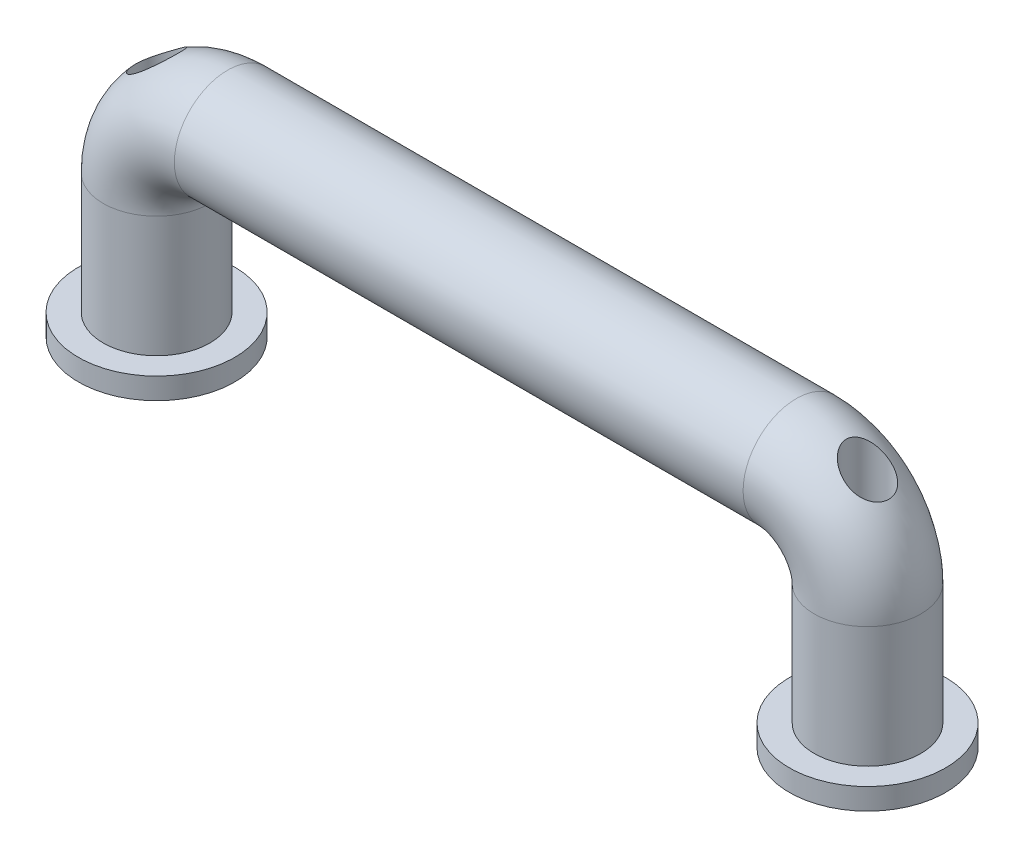
SolidWorks part; units mm, degrees
ref_plane "前视基准面" through (0, 0, 0) normal (0, 0, 1) x (1, 0, 0)
ref_plane "上视基准面" through (0, 0, 0) normal (0, 1, 0) x (1, 0, 0)
ref_plane "右视基准面" through (0, 0, 0) normal (1, 0, 0) x (0, 0, -1)
sketch "草图1" plane through (0, 0, 0) normal (0, 0, 1) x (1, 0, 0)
  line L0 (0, 0) -> (0, 20)
  line L1 (10, 30) -> (90, 30)
  line L2 (100, 20) -> (100, 0)
  arc A0 (0, 20) -> (10, 30) centre (10, 20) cw
  arc A1 (100, 20) -> (90, 30) centre (90, 20) ccw
  point P7 (0, 30)
  point P10 (100, 30)
  dimension "D3" = 10
  dimension "D4" = 10
  dimension "D1" = 30
  dimension "D2" = 100
sketch "草图2" plane through (0, 0, 0) normal (0, 1, 0) x (1, 0, 0)
  circle A0 centre (0, 0) radius 7.5
  dimension "D1" = 15
sweep "扫描1" add profiles "草图2" path "草图1"
sketch "草图3" plane through (0, 0, 0) normal (0, -1, 0) x (1, 0, 0)
  circle A0 centre (0, 0) radius 11
  circle A1 centre (100, 0) radius 11
  dimension "D1" = 22
extrude "凸台-拉伸1" add sketch "草图3" against normal blind 3
sketch "草图4" plane through (0, 0, 0) normal (0, -1, 0) x (1, 0, 0)
  circle A0 centre (0, 0) radius 1.65
  circle A1 centre (100, 0) radius 1.65
  dimension "D1" = 3.3
extrude "切除-拉伸1" cut sketch "草图4" against normal blind 51
sketch "草图5" plane through (0, 0, 0) normal (0, -1, 0) x (1, 0, 0)
  circle A0 centre (0, 0) radius 3
  circle A1 centre (100, 0) radius 3
  dimension "D1" = 6
extrude "切除-拉伸2" cut sketch "草图5" against normal blind 51 from offset 20
